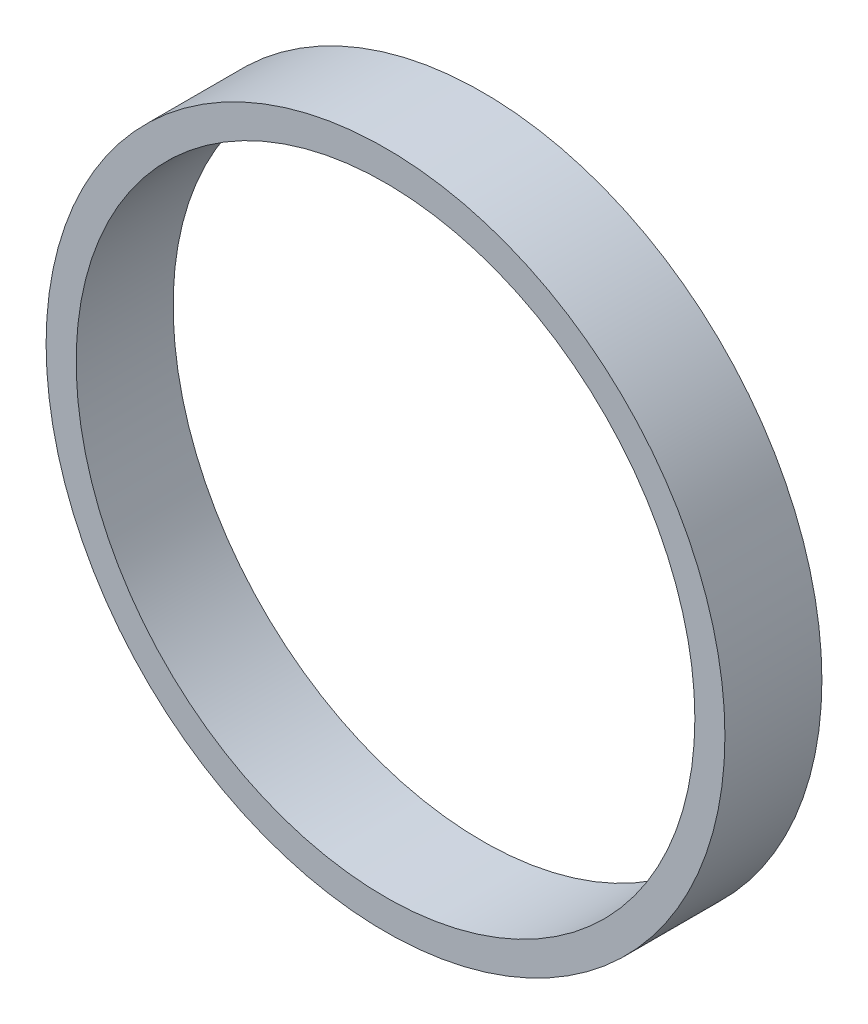
SolidWorks part; units mm, degrees
ref_plane "Front Plane" through (0, 0, 0) normal (0, 0, 1) x (1, 0, 0)
ref_plane "Top Plane" through (0, 0, 0) normal (0, 1, 0) x (1, 0, 0)
ref_plane "Right Plane" through (0, 0, 0) normal (1, 0, 0) x (0, 0, -1)
sketch "Sketch1" plane through (0, 0, 0) normal (0, 0, 1) x (1, 0, 0)
  circle A0 centre (0, 0) radius 175
  circle A1 centre (0, 0) radius 159.5
  dimension "D1" = 350
  dimension "D2" = 319
extrude "Boss-Extrude1" add sketch "Sketch1" along normal mid plane 50
